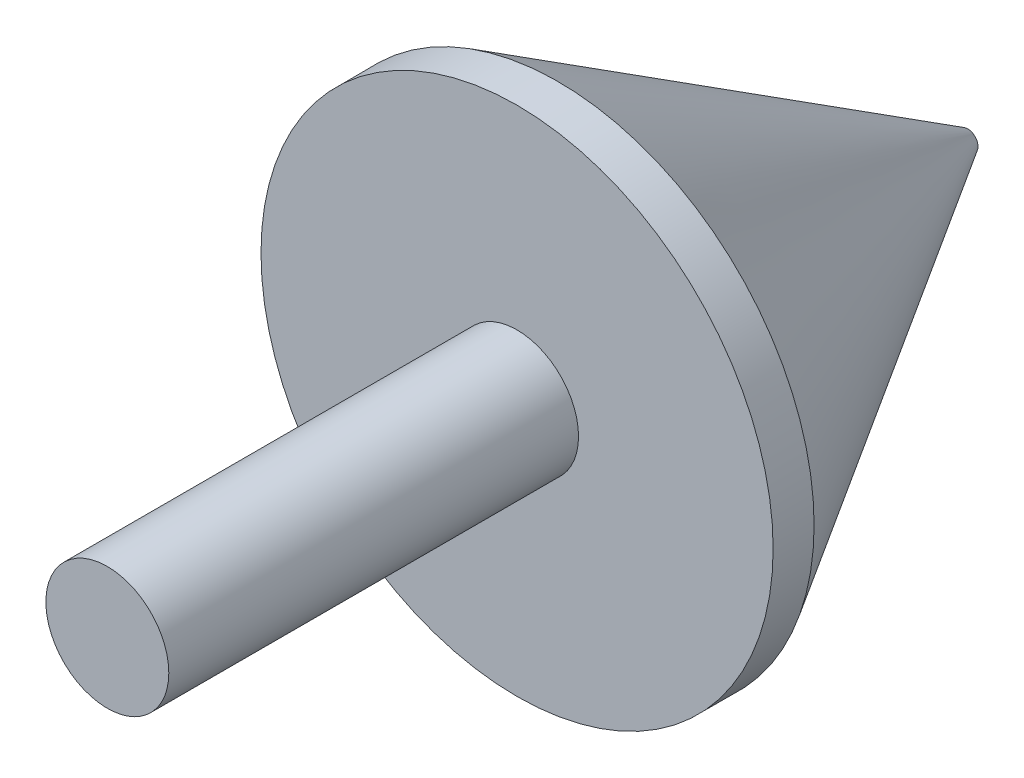
from build123d import *

# Parameters (mm, degrees)
SKETCH1_R           = 3
BOSS_EXTRUDE1_DEPTH = 20
SKETCH2_R           = 12.5
BOSS_EXTRUDE2_DEPTH = 2


with BuildPart() as part:
    # Sketch1 → Boss-Extrude1 (new body)
    with BuildSketch(Plane.XY):
        Circle(SKETCH1_R)
    extrude(amount=BOSS_EXTRUDE1_DEPTH)

    # Sketch2 → Boss-Extrude2 (add)
    with BuildSketch(Plane(origin=(0, 0, 0), x_dir=(-1, 0, 0), z_dir=(0, 0, -1))):
        Circle(SKETCH2_R)
    extrude(amount=BOSS_EXTRUDE2_DEPTH)

    # Sketch3 → Revolve2 (revolve)
    with BuildSketch(Plane(origin=(0, 0, 0), x_dir=(1, 0, 0), z_dir=(0, 1, 0)), mode=Mode.PRIVATE) as revolve2_sk:
        Polygon((-12.5, 2), (-0.5, 22), (0, 22), (0, 2), align=None)
    revolve(revolve2_sk.sketch.rotate(Axis((0, 0, -22), (0, 0, 1)), 180), axis=Axis((0, 0, -22), (0, 0, 1)))


solid = part.part
